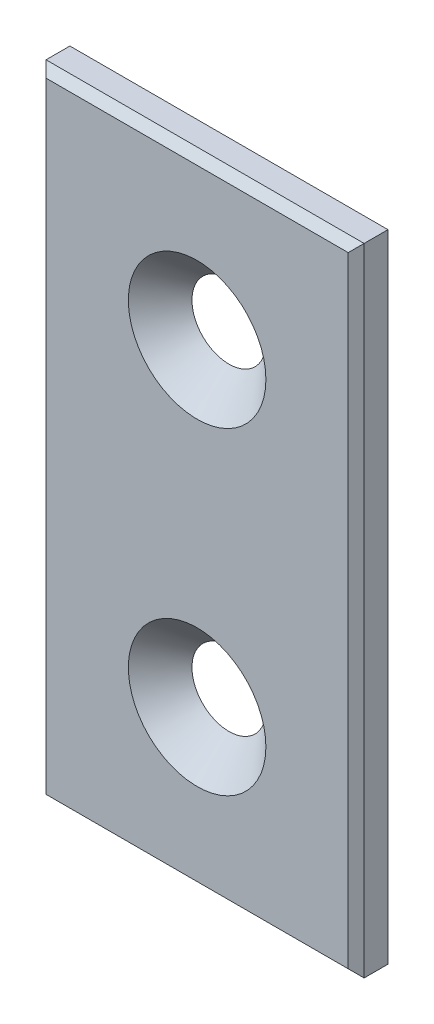
from build123d import *

# Parameters (mm, degrees)
SKETCH_1_W                = 40
SKETCH_1_H                = 80
EXTRUDE_1_DEPTH           = 2
HOLE_WIZARD_1_D           = 9
HOLE_WIZARD_1_DEPTH       = 10
HOLE_WIZARD_1_CSINK_D     = 17.3
HOLE_WIZARD_1_CSINK_ANGLE = 90
HOLE_WIZARD_1_TIP         = 2.703872786
CHAMFER_1_SIZE            = 1


with BuildPart() as part:
    # 草图1 → 凸台-拉伸1 (new, symmetric)
    with BuildSketch(Plane.XY):
        Rectangle(SKETCH_1_W, SKETCH_1_H)
    extrude(amount=EXTRUDE_1_DEPTH, both=True)

    # 打孔尺寸(%根据十字)槽沉头木螺钉的类型1
    with Locations(Plane(origin=(0, 20, 2), x_dir=(1, 0, 0), z_dir=(0, 0, 1))):
        with Locations((0, 0), (0, -40)):
            CounterSinkHole(HOLE_WIZARD_1_D / 2, HOLE_WIZARD_1_CSINK_D / 2, depth=HOLE_WIZARD_1_DEPTH, counter_sink_angle=HOLE_WIZARD_1_CSINK_ANGLE)
            with Locations((0, 0, -(HOLE_WIZARD_1_DEPTH + HOLE_WIZARD_1_TIP / 2))):  # 118° drill point
                Cone(0, HOLE_WIZARD_1_D / 2, HOLE_WIZARD_1_TIP, mode=Mode.SUBTRACT)

    # 倒角1
    chamfer_1_edges = [part.edges().sort_by_distance(p)[0] for p in [
        (-20, 0, 2),
        (0, -40, 2),
        (20, 0, 2),
        (0, 40, 2),
    ]]
    chamfer(chamfer_1_edges, length=CHAMFER_1_SIZE)


solid = part.part
